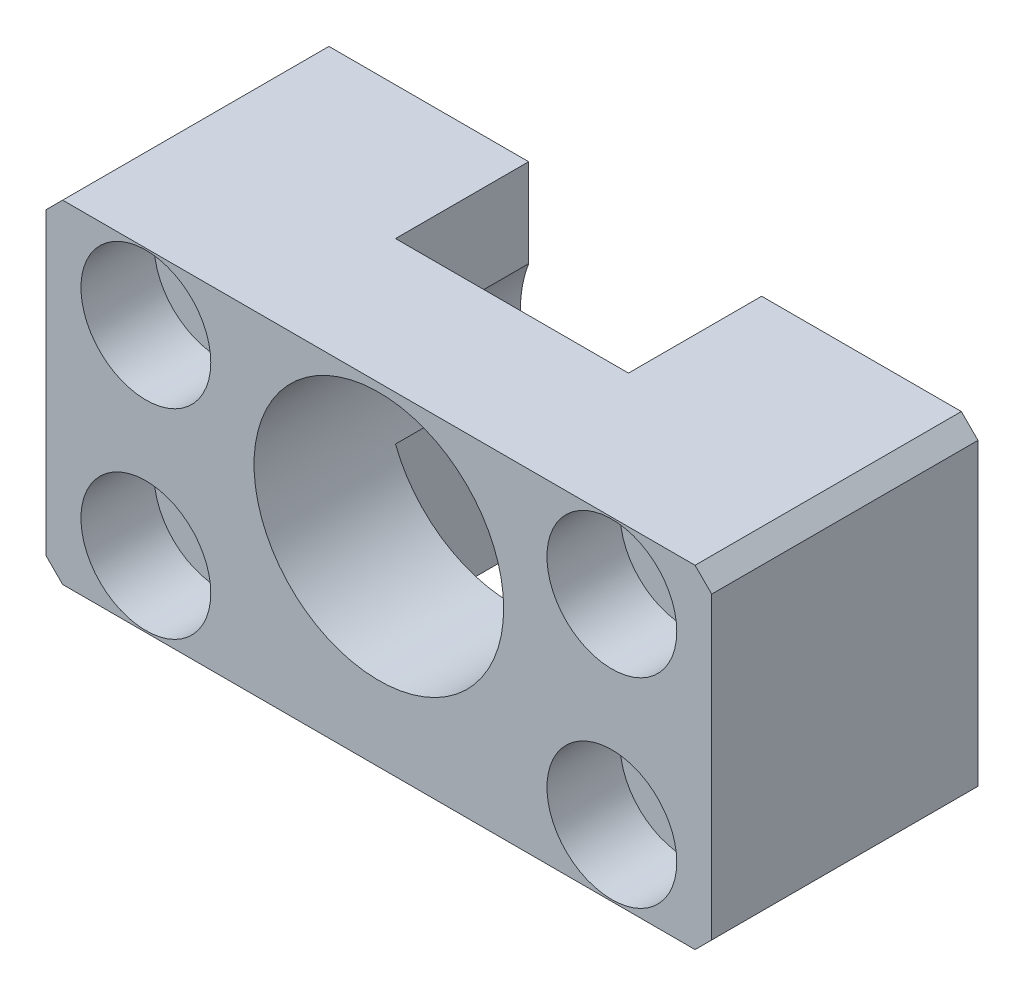
SolidWorks part; units mm, degrees
material "AL6061"
ref_plane "主视基准图" through (0, 0, 0) normal (0, 0, 1) x (1, 0, 0)
ref_plane "上视基准图" through (0, 0, 0) normal (0, 1, 0) x (1, 0, 0)
ref_plane "右视基准图" through (0, 0, 0) normal (1, 0, 0) x (0, 0, -1)
sketch "草图1" plane through (0, 0, 0) normal (0, 0, 1) x (1, 0, 0)
  line L1 (-20, -10) -> (20, -10)
  line L2 (-20, -10) -> (-20, 10)
  line L3 (-20, 10) -> (20, 10)
  line L4 (20, -10) -> (20, 10)
  line L5 (-20, -10) -> (20, 10) construction
  line L6 (-20, 10) -> (20, -10) construction
  point P0 (0, 0)
  dimension "D1" = 20
  dimension "D2" = 40
extrude "凸台-拉伸1" add sketch "草图1" along normal mid plane 16
chamfer "倒角1" distance 1 angle 45 4 edges at (-20, -10, 0) (20, -10, 0) (20, 10, 0) (-20, 10, 0)
hole_wizard "Ø15.0 (15) 直径孔1" positions "草图4" profile "草图3" hole size "Ø15.0" standard "Gb"
sketch "草图4" plane through (0, 0, 8) normal (0, 0, 1) x (1, 0, 0)
  line L0 (19, 10) -> (-19, 10) construction
  point P0 (0, 2)
  dimension "D1" = 8
sketch "草图3" plane through (0, 2, 8) normal (1, 0, 0) x (0, -1, 0)
  line L0 (0, 0) -> (0, 20)
  line L1 (0, 20) -> (7.5, 20)
  line L2 (7.5, 20) -> (7.5, 0)
  line L5 (7.5, 0) -> (0, 0)
  line L10 (0, 20) -> (-7.5, 20) construction
  line L11 (0, -6.35) -> (0, 107.95) construction
  dimension "孔直径" = 15
  dimension "孔深度" = 20
  dimension "导头角度" = 180
cosmetic thread "装饰螺纹线1" parameters "D2"=15.5
sketch "草图6" plane through (0, 0, -8) normal (0, 0, -1) x (-1, 0, 0)
  line L0 (-7, -14.9856) -> (-7, 13.1393)
  line L1 (7, -15.772) -> (7, 13.1393)
  line L2 (-7, 13.1393) -> (7, 13.1393)
  line L3 (0, 0) -> (0, 3.8058) construction
  line L4 (-7, -14.9856) -> (7, -15.772)
  circle A0 centre (0, 2) radius 7.5 construction
  dimension "D1" = 14
extrude "切除-拉伸2" cut sketch "草图6" against normal blind 8
hole_wizard "M4 六角凹头螺钉的柱形沉头孔3" positions "草图11" profile "草图9" counterbore size "M4" standard "Iso" end condition through all
sketch "草图11" plane through (0, 0, 8) normal (0, 0, 1) x (1, 0, 0)
  line L1 (-14, -6) -> (14, -6) construction
  line L2 (-14, -6) -> (-14, 6) construction
  line L3 (-14, 6) -> (14, 6) construction
  line L4 (14, -6) -> (14, 6) construction
  line L5 (-14, -6) -> (14, 6) construction
  line L6 (-14, 6) -> (14, -6) construction
  line L7 (0, 0) -> (0, 7.0783) construction
  line L8 (0, 0) -> (6.8535, 0) construction
  line L9 (-20, 9) -> (-20, -9) construction
  point P1 (0, 0)
  point P2 (14, 6)
  point P133 (-14, -6)
  point P134 (-14, 6)
  point P135 (14, -6)
  dimension "D1" = 12
  dimension "D2" = 6
sketch "草图9" plane through (0, 0, 8) normal (1, 0, 0) x (0, -1, 0)
  line L0 (0, 0) -> (0, 16)
  line L1 (0, 16) -> (2.25, 16)
  line L3 (2.25, 16) -> (2.25, 4.4)
  line L4 (2.25, 4.4) -> (3.9, 4.4)
  line L5 (3.9, 4.4) -> (3.9, 0)
  line L7 (3.9, 0) -> (0, 0)
  line L11 (0, -6.35) -> (0, 107.95) construction
  dimension "通孔孔直径" = 4.5
  dimension "通孔孔深度" = 16
  dimension "柱形沉头孔直径" = 7.8
  dimension "柱形沉头孔深度" = 4.4
